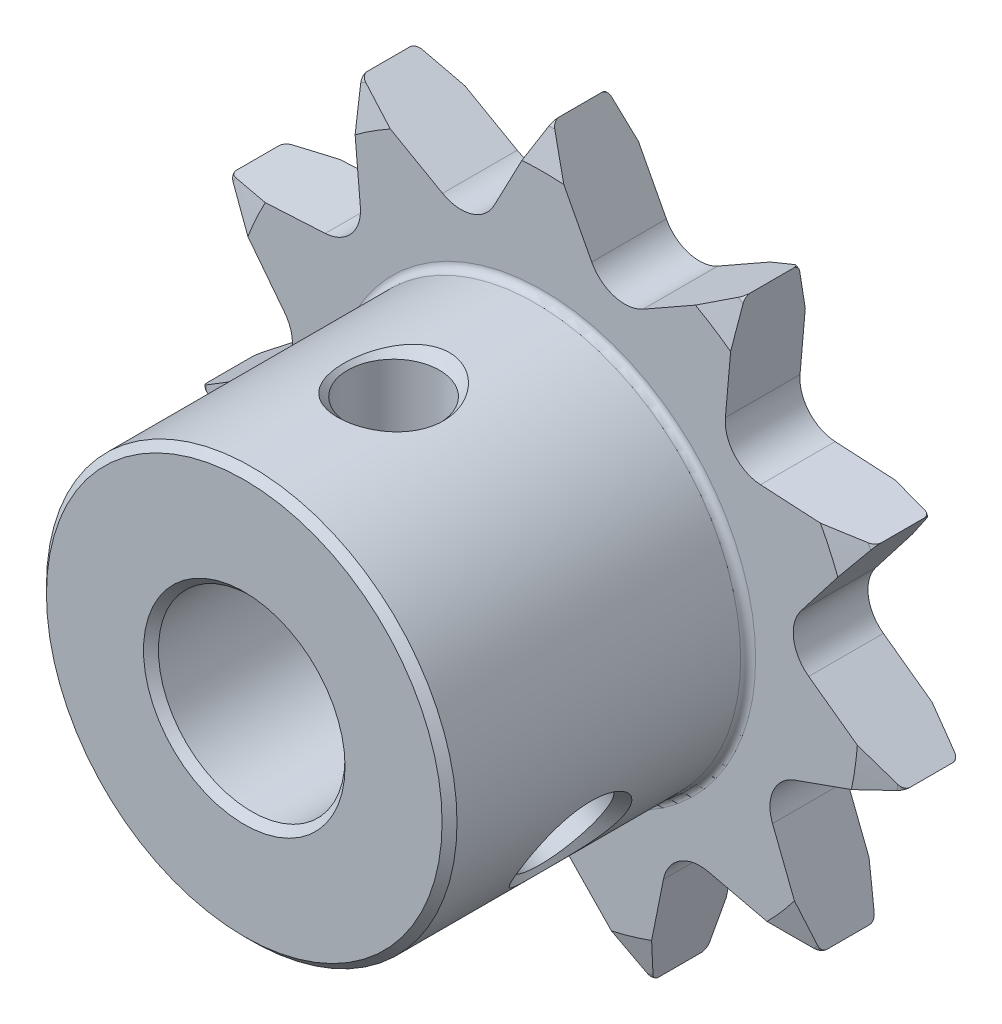
SolidWorks part; units mm, degrees
ref_plane "前视基准面" through (0, 0, 0) normal (0, 0, 1) x (1, 0, 0)
ref_plane "上视基准面" through (0, 0, 0) normal (0, 1, 0) x (1, 0, 0)
ref_plane "右视基准面" through (0, 0, 0) normal (1, 0, 0) x (0, 0, -1)
sketch "草图1" plane through (0, 0, 0) normal (1, 0, 0) x (0, 0, -1)
  line L0 (-10, 2.7) -> (-9.8, 2.5)
  line L1 (-9.8, 2.5) -> (-0.2, 2.5)
  line L2 (-0.2, 2.5) -> (0, 2.7)
  line L3 (0, 2.7) -> (0, 8.45)
  line L4 (0, 8.45) -> (-0.2416, 9.3518)
  line L5 (-0.4348, 9.5) -> (-1.5652, 9.5)
  line L6 (-1.7584, 9.3518) -> (-2, 8.45)
  line L7 (-2, 8.45) -> (-2, 5.7)
  line L8 (-2.2, 5.5) -> (-9.8, 5.5)
  line L9 (-9.8, 5.5) -> (-10, 5.3)
  line L10 (-10, 5.3) -> (-10, 2.7)
  line L11 (0, 0) -> (-10, 0) construction
  arc A0 (-0.2416, 9.3518) -> (-0.4348, 9.5) centre (-0.4348, 9.3) ccw
  arc A1 (-1.5652, 9.5) -> (-1.7584, 9.3518) centre (-1.5652, 9.3) ccw
  arc A2 (-2, 5.7) -> (-2.2, 5.5) centre (-2.2, 5.7) cw
revolve "旋转1" add sketch "草图1" angle 360 about L11
sketch "草图2" plane through (0, 0, 0) normal (0, 0, 1) x (1, 0, 0)
  line L0 (-150.3101, -119.3707) -> (151.6954, -119.3707)
  line L1 (151.6954, -119.3707) -> (151.6954, 126.7592)
  line L2 (151.6954, 126.7592) -> (-150.3101, 126.7592)
  line L3 (-150.3101, 126.7592) -> (-150.3101, -119.3707)
  line L4 (-9.4033, -1.352) -> (-6.7499, -2.2927)
  line L5 (-6.1529, -3.5999) -> (-7.1796, -6.2212)
  line L6 (-7.1796, -6.2212) -> (-4.4389, -5.578)
  line L7 (-3.2299, -6.3549) -> (-2.6765, -9.1152)
  line L8 (-2.6765, -9.1152) -> (-0.7185, -7.0924)
  line L9 (0.7185, -7.0924) -> (2.6765, -9.1152)
  line L10 (2.6765, -9.1152) -> (3.2299, -6.3549)
  line L11 (4.4389, -5.578) -> (7.1796, -6.2212)
  line L12 (7.1796, -6.2212) -> (6.1529, -3.5999)
  line L13 (6.7499, -2.2927) -> (9.4033, -1.352)
  line L14 (9.4033, -1.352) -> (7.1224, 0.2981)
  line L15 (6.9179, 1.7206) -> (8.6415, 3.9464)
  line L16 (8.6415, 3.9464) -> (5.8306, 4.1015)
  line L17 (4.8895, 5.1875) -> (5.1361, 7.9919)
  line L18 (5.1361, 7.9919) -> (2.6876, 6.6026)
  line L19 (1.3087, 7.0075) -> (0, 9.5)
  line L20 (0, 9.5) -> (-1.3087, 7.0075)
  line L21 (-2.6876, 6.6026) -> (-5.1361, 7.9919)
  line L22 (-5.1361, 7.9919) -> (-4.8895, 5.1875)
  line L23 (-5.8306, 4.1015) -> (-8.6415, 3.9464)
  line L24 (-8.6415, 3.9464) -> (-6.9179, 1.7206)
  line L25 (-7.1224, 0.2981) -> (-9.4033, -1.352)
  arc A0 (-6.7499, -2.2927) -> (-6.1529, -3.5999) centre (-7.0841, -3.2352) cw
  arc A1 (-4.4389, -5.578) -> (-3.2299, -6.3549) centre (-4.2104, -6.5516) cw
  arc A2 (-0.7185, -7.0924) -> (0.7185, -7.0924) centre (0, -7.7878) cw
  arc A3 (3.2299, -6.3549) -> (4.4389, -5.578) centre (4.2104, -6.5516) cw
  arc A4 (6.1529, -3.5999) -> (6.7499, -2.2927) centre (7.0841, -3.2352) cw
  arc A5 (7.1224, 0.2981) -> (6.9179, 1.7206) centre (7.7086, 1.1083) cw
  arc A6 (5.8306, 4.1015) -> (4.8895, 5.1875) centre (5.8857, 5.1) cw
  arc A7 (2.6876, 6.6026) -> (1.3087, 7.0075) centre (2.1941, 7.4724) cw
  arc A8 (-1.3087, 7.0075) -> (-2.6876, 6.6026) centre (-2.1941, 7.4724) cw
  arc A9 (-4.8895, 5.1875) -> (-5.8306, 4.1015) centre (-5.8857, 5.1) cw
  arc A10 (-6.9179, 1.7206) -> (-7.1224, 0.2981) centre (-7.7086, 1.1083) cw
extrude "切除-拉伸1" cut sketch "草图2" along normal blind 2
ref_plane "基准面4" through (0, 0, 6) normal (0, 0, 1) x (1, 0, 0)
sketch "草图3" plane through (0, 0, 6) normal (0, 0, 1) x (1, 0, 0)
  line L0 (0, 0) -> (-1.5, 0)
  line L1 (-1.5, 0) -> (-1.5, 2.5)
  line L2 (-1.5, 2.5) -> (-1.2295, 2.7705)
  line L3 (-1.2295, 2.7705) -> (-1.2295, 5.2295)
  line L4 (-1.2295, 5.2295) -> (-1.5, 5.5)
  line L5 (-1.5, 5.5) -> (-1.5, 8)
  line L6 (-1.5, 8) -> (0, 8)
  line L7 (0, 8) -> (0, 0)
  line L8 (0, 5.5) -> (0, 2.5) construction
revolve "切除-旋转1" cut sketch "草图3" angle 360 about L8
cosmetic thread "装饰螺纹线1" parameters "D1"=2.7295, "D2"=3
sketch "草图4" plane through (0, 0, 6) normal (0, 0, 1) x (1, 0, 0)
  line L0 (0, 0) -> (0.75, 1.299)
  line L1 (0.75, 1.299) -> (2.9151, 0.049)
  line L2 (2.9151, 0.049) -> (3.0141, -0.3205)
  line L3 (3.0141, -0.3205) -> (5.1436, -1.55)
  line L4 (5.1436, -1.55) -> (5.5131, -1.451)
  line L5 (5.5131, -1.451) -> (7.6782, -2.701)
  line L6 (7.6782, -2.701) -> (6.9282, -4)
  line L7 (6.9282, -4) -> (0, 0)
  line L8 (4.7631, -2.75) -> (2.1651, -1.25) construction
revolve "切除-旋转2" cut sketch "草图4" angle 360 about L8
cosmetic thread "装饰螺纹线2" parameters "D1"=2.7295, "D2"=3
